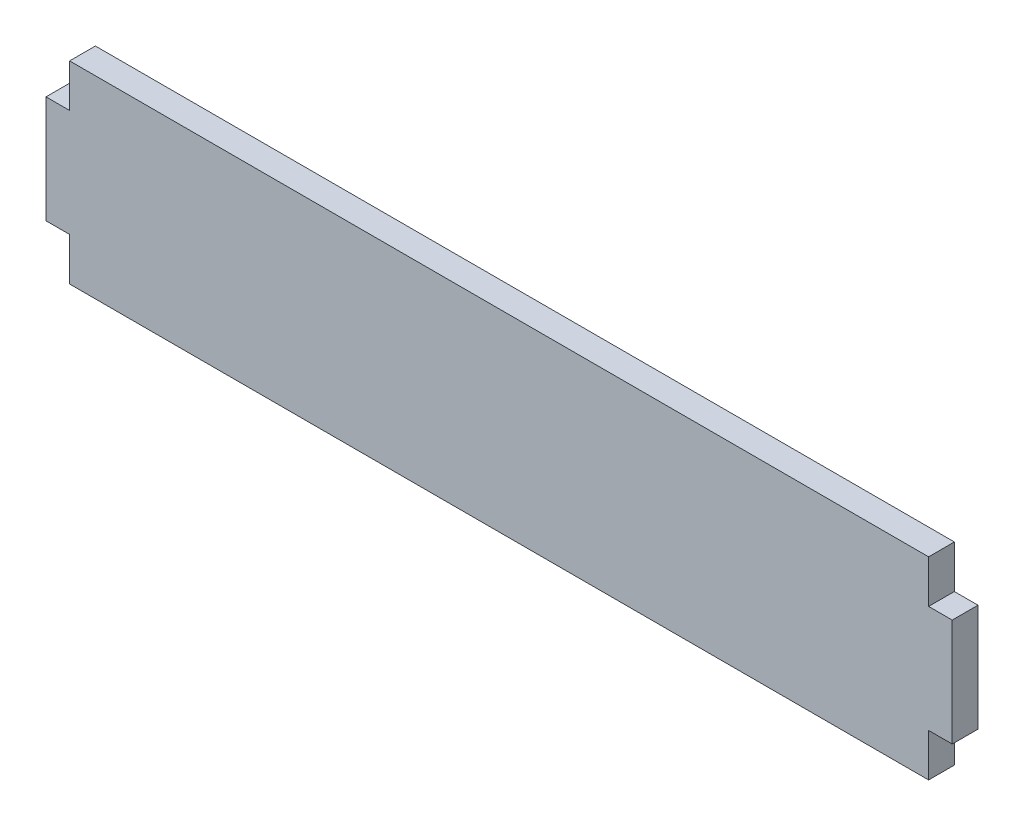
SolidWorks part; units mm, degrees
material "SS400P"
ref_plane "Front Plane" through (0, 0, 0) normal (0, 0, 1) x (1, 0, 0)
ref_plane "Top Plane" through (0, 0, 0) normal (0, 1, 0) x (1, 0, 0)
ref_plane "Right Plane" through (0, 0, 0) normal (1, 0, 0) x (0, 0, -1)
sketch "Sketch1" plane through (0, 0, 0) normal (0, 0, 1) x (1, 0, 0)
  line L0 (43.6, -110) -> (-156.4, -110)
  line L1 (-156.4, -110) -> (-156.4, -100)
  line L2 (-156.4, -110) -> (-156.4, 100) construction
  line L3 (-156.4, -65) -> (43.6, -65)
  line L5 (43.6, 100) -> (43.6, -110) construction
  line L6 (43.6, -65) -> (43.6, -75)
  line L7 (-156.4, -100) -> (-161.9, -100)
  line L8 (-161.9, -100) -> (-161.9, -75)
  line L9 (-161.9, -75) -> (-156.4, -75)
  line L10 (-156.4, -75) -> (-156.4, -65)
  line L11 (43.6, -100) -> (49.1, -100)
  line L12 (49.1, -100) -> (49.1, -75)
  line L13 (49.1, -75) -> (43.6, -75)
  line L14 (43.6, -100) -> (43.6, -110)
  dimension "D1" = 45
  dimension "D2" = 5.5
  dimension "D3" = 25
  dimension "D4" = 5.5
  dimension "D5" = 25
extrude "Boss-Extrude1" add sketch "Sketch1" along normal mid plane 6
